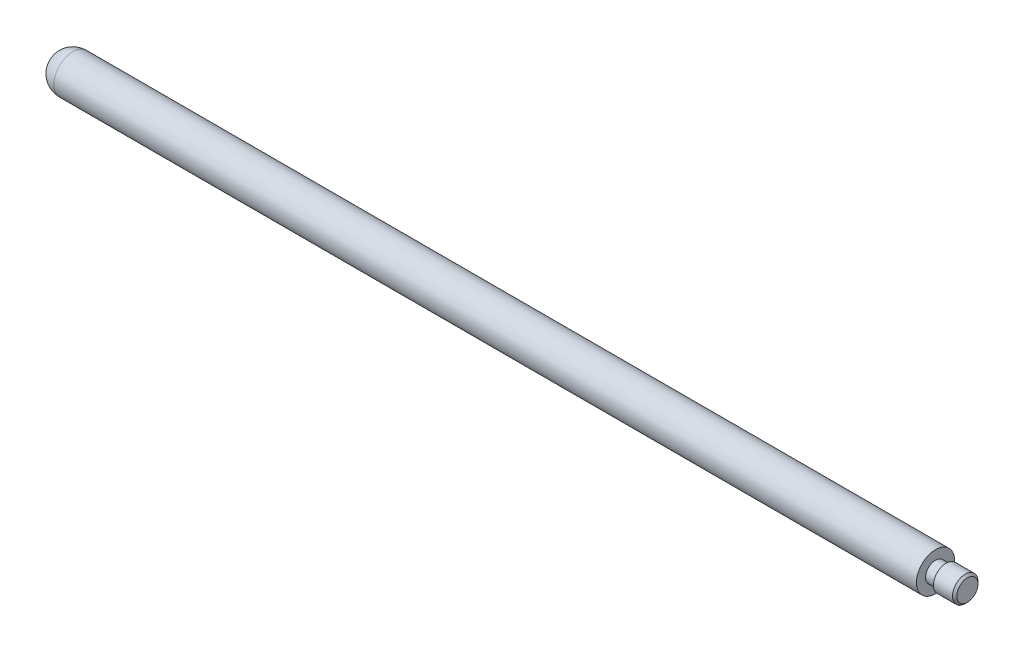
SolidWorks part; units mm, degrees
ref_plane "Front Plane" through (0, 0, 0) normal (0, 0, 1) x (1, 0, 0)
ref_plane "Top Plane" through (0, 0, 0) normal (0, 1, 0) x (1, 0, 0)
ref_plane "Right Plane" through (0, 0, 0) normal (1, 0, 0) x (0, 0, -1)
sketch "Sketch1" plane through (0, 0, 0) normal (0, 0, 1) x (1, 0, 0)
  line L7 (-15, 0) -> (-15, 4.7) construction
  line L8 (0, 0) -> (-10, 0)
  line L9 (0, 0) -> (0, 6)
  line L10 (0, 6) -> (-10, 6)
  line L11 (-10, 4.7) -> (-10, 6)
  line L12 (-10, 0) -> (-15, 0)
  line L13 (-10, 0) -> (-10, 4.7) construction
  line L14 (-10, 4.7) -> (-15, 4.7)
  line L15 (-15, 0) -> (-15, 4.7) construction
  line L16 (-15, 0) -> (-430, 0)
  line L17 (-15, 4.7) -> (-15, 9)
  line L18 (-15, 9) -> (-421, 9)
  line L20 (-10, 0) -> (-10, 4.7) construction
  arc A1 (-421, 9) -> (-430, 0) centre (-421, 0) ccw
  dimension "D2" = 10
  dimension "D4" = 5
  dimension "D7" = 18
  dimension "D1" = 6
  dimension "D3" = 4.7
  dimension "D5" = 9
  dimension "D6" = 415
revolve "Revolve2" add sketch "Sketch1" angle 360 about L16
cosmetic thread "Cosmetic Thread1" parameters "D2"=10.106
chamfer "Chamfer1" distance 1 angle 45 1 edges at (0, 0, -6)
